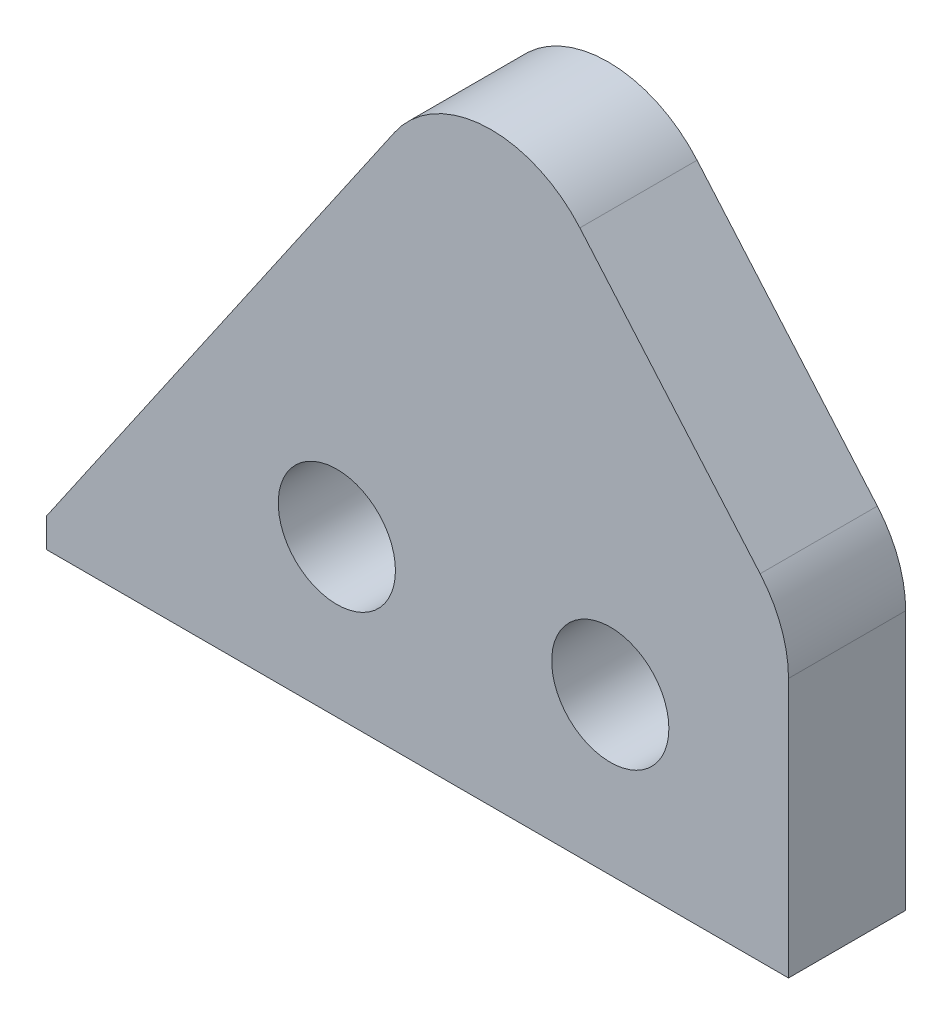
from build123d import *

# Parameters (mm, degrees)
SKETCH1_R           = 15
BOSS_EXTRUDE1_DEPTH = 30


with BuildPart() as part:
    # Sketch1 → Boss-Extrude1 (new body)
    with BuildSketch(Plane.XY):
        with BuildLine():
            Line((137442.792186055, -173144.918087479), (137353.659547419, -173274.56556186))
            Line((137353.659547419, -173274.56556186), (137353.659547419, -173281.943182873))
            Line((137353.659547419, -173281.943182873), (137543.659547419, -173281.943182873))
            Line((137543.659547419, -173281.943182873), (137543.659547419, -173215.524161381))
            ThreePointArc((137543.659547419, -173215.524161381), (137541.785217916, -173205.086409641), (137536.396436674, -173195.952910355))
            Line((137536.396436674, -173195.952910355), (137490.250333171, -173142.34270129))
            ThreePointArc((137490.250333171, -173142.34270129), (137465.887841454, -173131.958027607), (137442.792186055, -173144.918087479))
        make_face()
        with Locations((137498.03455904, -173241.943182873)):
            Circle(SKETCH1_R, mode=Mode.SUBTRACT)
        with Locations((137428.03455904, -173241.943182873)):
            Circle(SKETCH1_R, mode=Mode.SUBTRACT)
    extrude(amount=BOSS_EXTRUDE1_DEPTH)


solid = part.part
